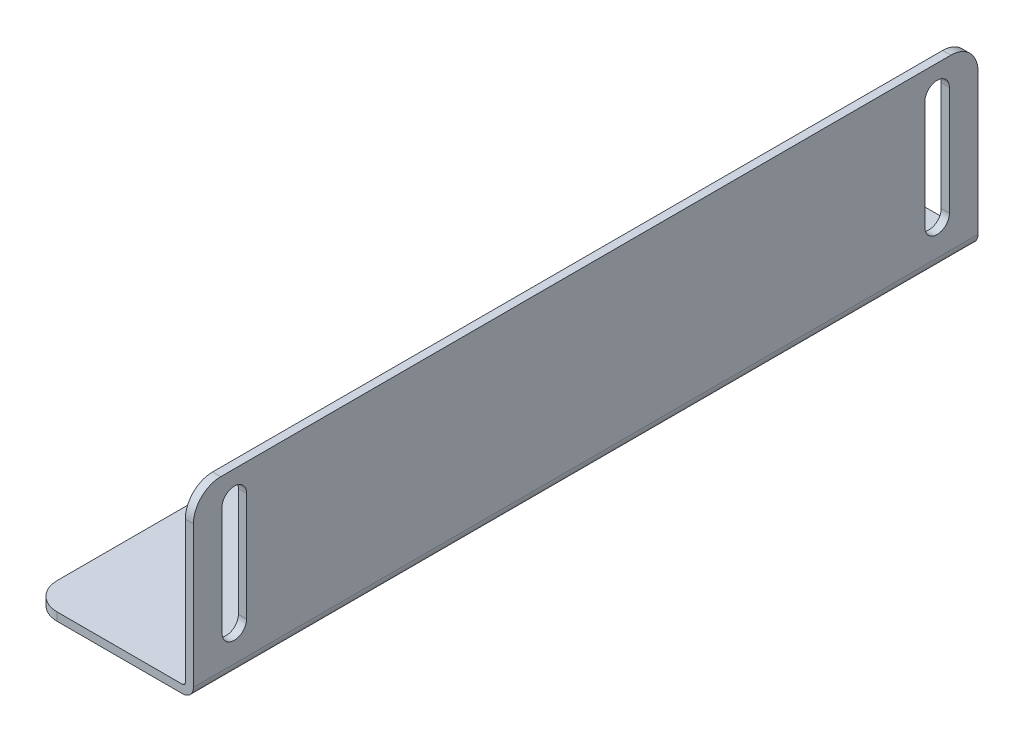
SolidWorks part; units mm, degrees
material "1.5不锈钢"
ref_plane "Front" through (0, 0, 0) normal (0, 0, 1) x (1, 0, 0)
ref_plane "Top" through (0, 0, 0) normal (0, 1, 0) x (1, 0, 0)
ref_plane "Right" through (0, 0, 0) normal (1, 0, 0) x (0, 0, -1)
sketch "草图1" plane through (0, 0, 0) normal (0, 0, 1) x (1, 0, 0)
  line L0 (0, 0) -> (30, 0)
  line L1 (0, 0) -> (0, 33)
  line L2 (0, 33) -> (30, 33)
  line L4 (30, 33) -> (30, 0)
  dimension "D3" = 30
  dimension "D4" = 33
extrude "凸台-拉伸1" add sketch "草图1" along normal blind 144
shell "抽壳1" thickness 1.5
fillet "圆角1" radius 5 4 edges at (0, 0.75, 144) (29.25, 33, 144) (29.25, 33, 0) (0, 0.75, 0)
fillet "圆角2" radius 0.5 1 edges at (28.5, 1.5, 72)
fillet "圆角3" radius 2 1 edges at (30, 0, 72)
sketch "草图2" plane through (28.5, 0, -49) normal (-1, 0, 0) x (0, 0, 1)
  line L0 (56.5, 8) -> (56.5, 28) construction
  line L1 (54.25, 8) -> (54.25, 28)
  line L2 (58.75, 8) -> (58.75, 28)
  line L3 (49, 2) -> (49, 28) construction
  line L5 (188, 33) -> (54, 33) construction
  line L6 (185.5, 28) -> (185.5, 8) construction
  line L8 (187.75, 28) -> (187.75, 8)
  line L9 (183.25, 28) -> (183.25, 8)
  line L10 (193, 2) -> (193, 28) construction
  arc A0 (54.25, 8) -> (58.75, 8) centre (56.5, 8) ccw
  arc A1 (58.75, 28) -> (54.25, 28) centre (56.5, 28) ccw
  arc A2 (187.75, 28) -> (183.25, 28) centre (185.5, 28) ccw
  arc A3 (183.25, 8) -> (187.75, 8) centre (185.5, 8) ccw
  point P2 (56.5, 18)
  point P13 (185.5, 18)
  dimension "D2" = 2.25
  dimension "D3" = 5
  dimension "D6" = 5
  dimension "D1" = 7.5
  dimension "D4" = 20
  dimension "D5" = 7.5
extrude "切除-拉伸1" cut sketch "草图2" against normal through all
sketch "草图3" plane through (0, 0, 0) normal (0, 1, 0) x (1, 0, 0)
  line L2 (30, -139) -> (30, -5) construction
  line L4 (0, -72) -> (28.1433, -72) construction
  line L5 (0, -139) -> (0, -5) construction
  circle A0 centre (5, -87.875) radius 1.75
  circle A2 centre (5, -56.125) radius 1.75
  dimension "D1" = 3.5
  dimension "D2" = 25
  dimension "D5" = 31.75
extrude "切除-拉伸2" cut sketch "草图3" along normal up to next
sketch "草图4" plane through (0, 0, 0) normal (0, 1, 0) x (1, 0, 0)
  line L0 (5, -100.375) -> (5, -75.375) construction
  line L1 (3.25, -100.375) -> (3.25, -75.375)
  line L2 (6.75, -100.375) -> (6.75, -75.375)
  line L3 (5, -68.625) -> (5, -43.625) construction
  line L4 (3.25, -68.625) -> (3.25, -43.625)
  line L5 (6.75, -68.625) -> (6.75, -43.625)
  arc A0 (3.25, -100.375) -> (6.75, -100.375) centre (5, -100.375) ccw
  arc A1 (6.75, -75.375) -> (3.25, -75.375) centre (5, -75.375) ccw
  arc A2 (3.25, -68.625) -> (6.75, -68.625) centre (5, -68.625) ccw
  arc A3 (6.75, -43.625) -> (3.25, -43.625) centre (5, -43.625) ccw
  circle A6 centre (5, -87.875) radius 1.75 construction
  circle A7 centre (5, -56.125) radius 1.75 construction
  point P3 (5, -87.875)
  point P8 (5, -56.125)
  dimension "D1" = 3.5
  dimension "D2" = 25
extrude "切除-拉伸3" cut sketch "草图4" along normal up to next
